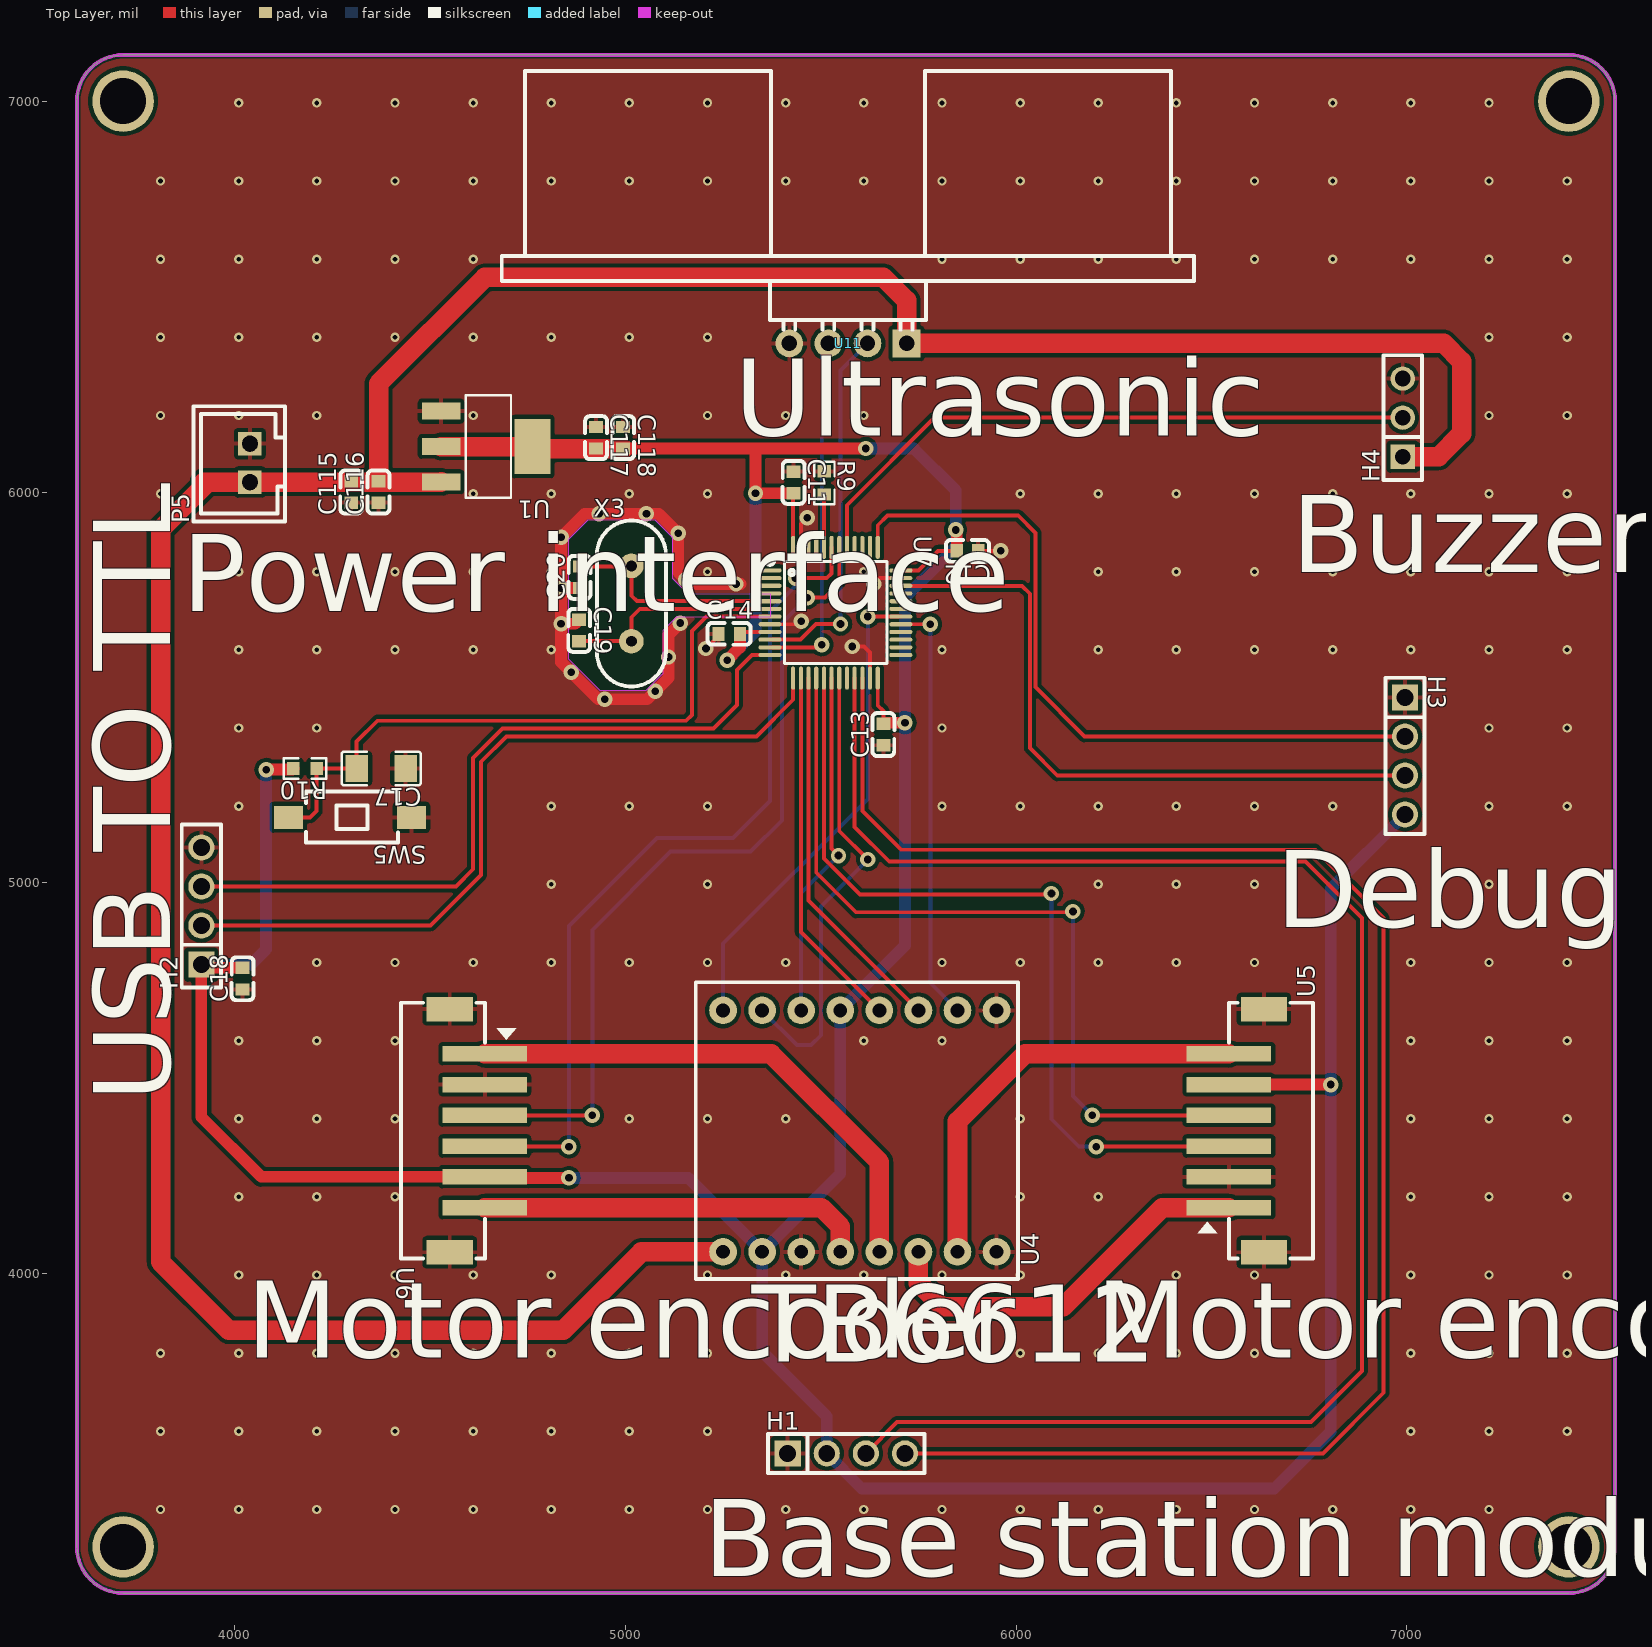
[diagram p0: Top Layer view]
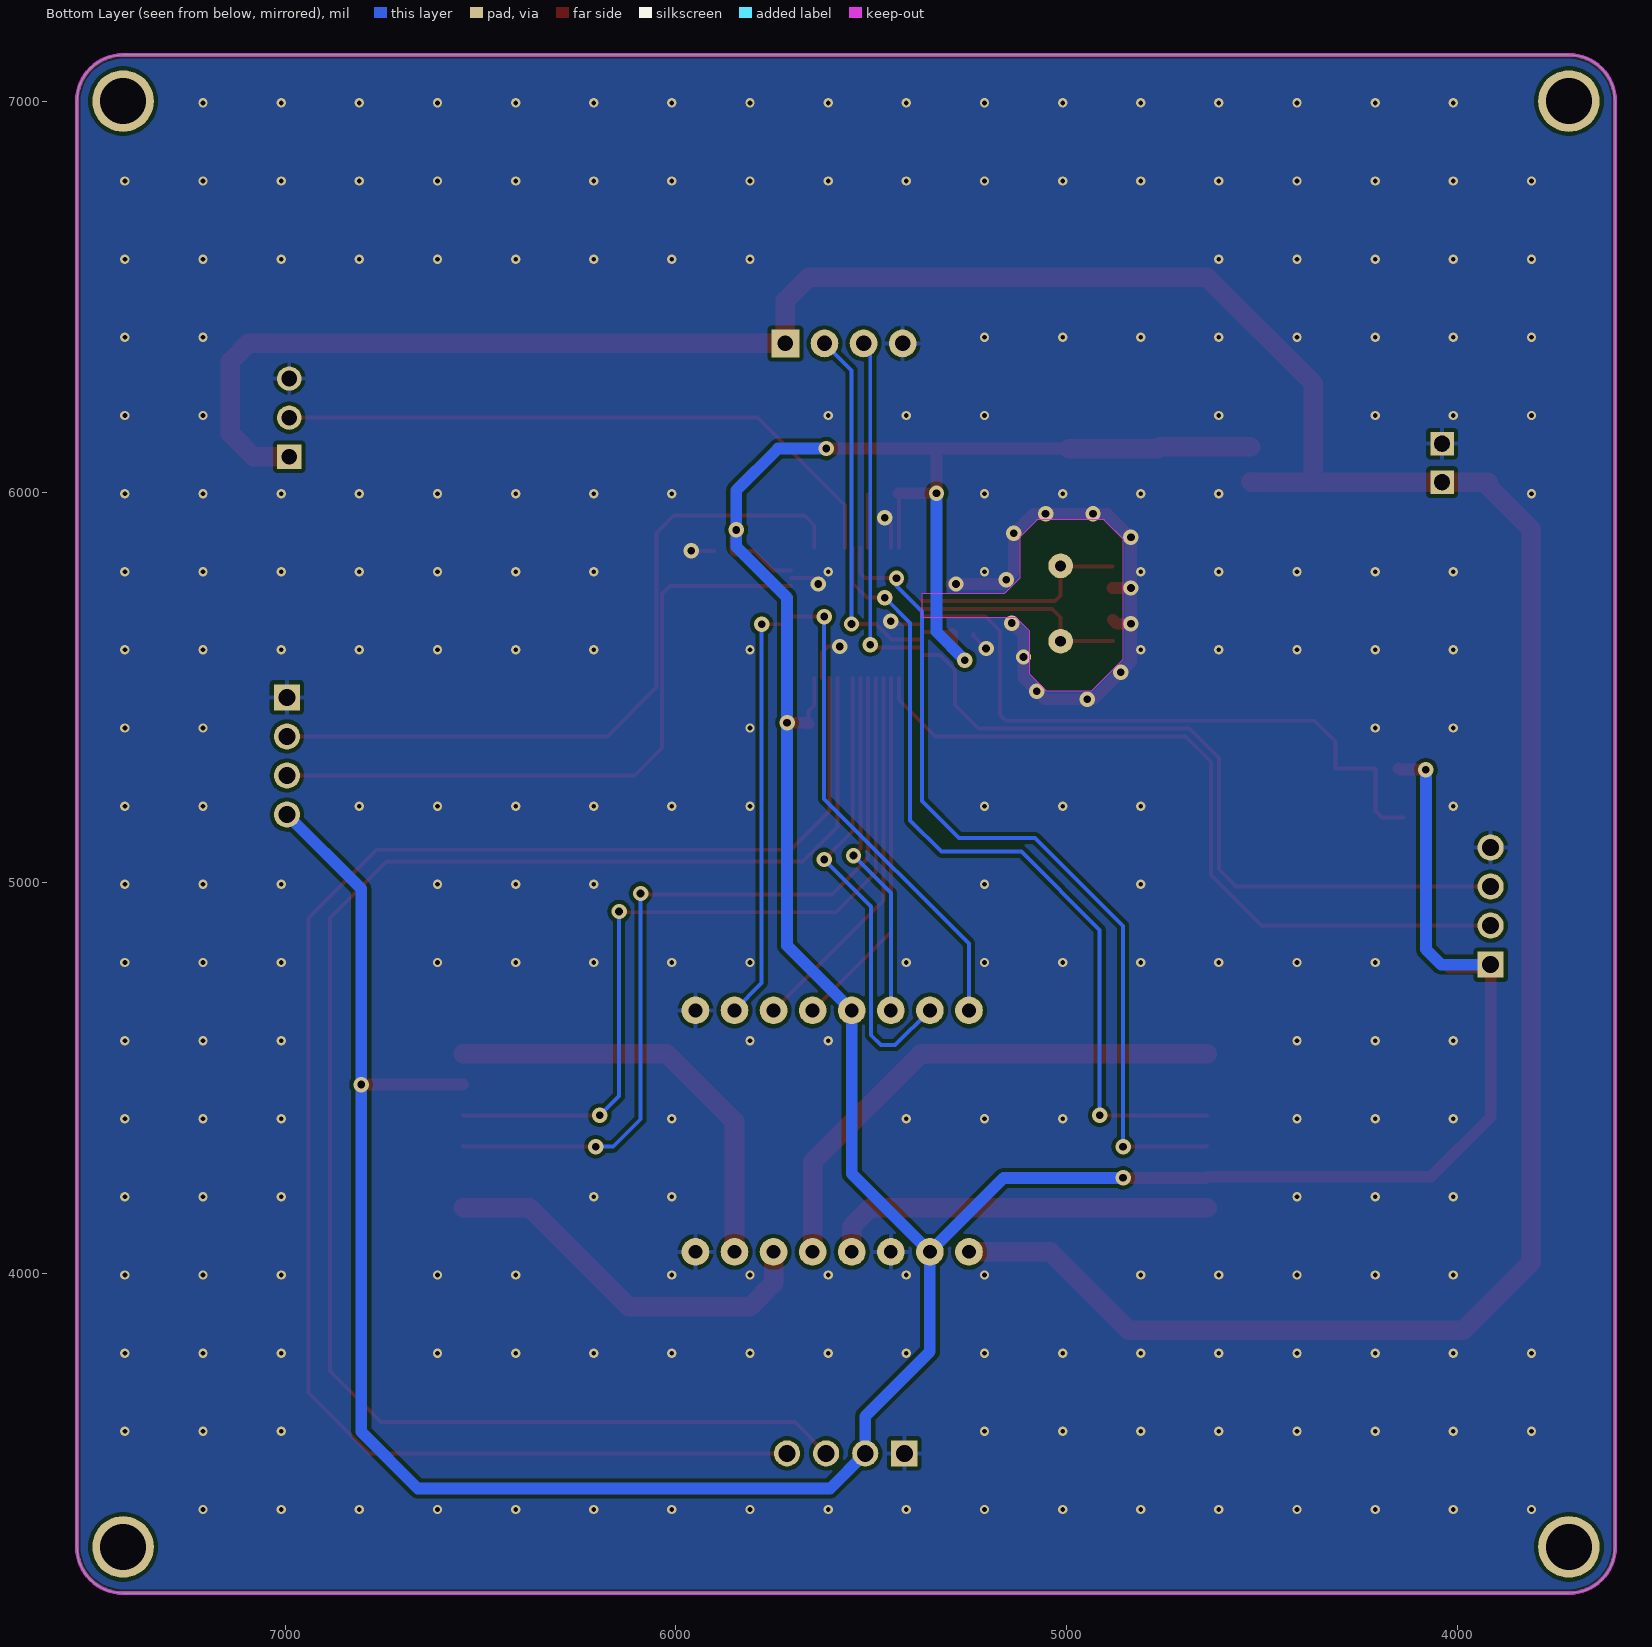
[diagram p1: Bottom Layer view, seen from below]
# Altium PCB MISC61262.pcbdoc
Units mil, origin at the board's own origin, x right, y up, seen from the top; angles counter-clockwise.
Board outline 3937.01 x 3937.01 mil, 2 copper layers (Top Layer, Bottom Layer), stack 62.206 mil thick; 27 components, 45 nets, 141 pads, 278 vias.

## Layer stack, top to bottom
Top Solder Mask Layer: solder mask 0.394, Dk 3.3
Top Layer: signal copper 1.379
Dielectric1: surface 59.449, FR4, Dk 4.5
Bottom Layer: signal copper 1.378
Bottom Solder Mask Layer: solder mask 0.394, Dk 3.3

## Board outline
3595.71,3300.39 ccw(c3713.82,3300.39) 3713.82,3182.28 7414.61,3182.28 ccw(c7414.61,3300.39) 7532.72,3300.39 7532.72,7001.18 ccw(c7414.61,7001.18) 7414.61,7119.29 3713.82,7119.29 ccw(c3713.82,7001.18) 3595.71,7001.18

## Design rules (kind name [scope] priority, off if disabled: settings)
BoardOutlineClearance copperThickness2oz_1 [All] p2 off: genericclearance=7.99 ignorepadtopadclearanceinfootprint=FALSE except(0: Arc-SplitContinuation Track-SplitContinuation SMDPad-SplitContinuation THPad-SplitContinuation Via-SplitContinuation Fill-SplitContinuation Region-SplitContinuation Poly-SplitContinuation Text-SplitContinuation Hole-SplitContinuation; 5.98: Arc-CutoutEdge Track-CutoutEdge SMDPad-CutoutEdge THPad-CutoutEdge Via-CutoutEdge Text-CutoutEdge; 6.9: Hole-OutlineEdge Hole-CutoutEdge; 10: Poly-OutlineEdge Poly-CutoutEdge; 11.81: Arc-OutlineEdge Track-OutlineEdge SMDPad-OutlineEdge THPad-OutlineEdge Via-OutlineEdge Fill-OutlineEdge Region-OutlineEdge Text-OutlineEdge Fill-CutoutEdge Region-CutoutEdge)
BoardOutlineClearance Plane_innerPlane_1 [All] p4 off: genericclearance=4.02 ignorepadtopadclearanceinfootprint=FALSE except(0: Arc-SplitContinuation Track-SplitContinuation SMDPad-SplitContinuation THPad-SplitContinuation Via-SplitContinuation Fill-SplitContinuation Region-SplitContinuation Poly-SplitContinuation Text-SplitContinuation Hole-SplitContinuation; 5.98: Arc-CutoutEdge Track-CutoutEdge SMDPad-CutoutEdge THPad-CutoutEdge Via-CutoutEdge Text-CutoutEdge; 6.9: Hole-OutlineEdge Hole-CutoutEdge; 10: Poly-OutlineEdge Poly-CutoutEdge; 11.81: Arc-OutlineEdge Track-OutlineEdge SMDPad-OutlineEdge THPad-OutlineEdge Via-OutlineEdge Fill-OutlineEdge Region-OutlineEdge Text-OutlineEdge Fill-CutoutEdge Region-CutoutEdge)
BoardOutlineClearance Copper_copperRegion_1 [All] p6 off: genericclearance=4.02 ignorepadtopadclearanceinfootprint=FALSE except(0: Arc-SplitContinuation Track-SplitContinuation SMDPad-SplitContinuation THPad-SplitContinuation Via-SplitContinuation Fill-SplitContinuation Region-SplitContinuation Poly-SplitContinuation Text-SplitContinuation Hole-SplitContinuation; 5.98: Arc-CutoutEdge Track-CutoutEdge SMDPad-CutoutEdge THPad-CutoutEdge Via-CutoutEdge Text-CutoutEdge; 6.9: Hole-OutlineEdge Hole-CutoutEdge; 10: Poly-OutlineEdge Poly-CutoutEdge; 11.81: Arc-OutlineEdge Track-OutlineEdge SMDPad-OutlineEdge THPad-OutlineEdge Via-OutlineEdge Fill-OutlineEdge Region-OutlineEdge Text-OutlineEdge Fill-CutoutEdge Region-CutoutEdge)
BoardOutlineClearance Copper_copperRegion_copperThickness1oz_1 [All] p8 off: genericclearance=4.02 ignorepadtopadclearanceinfootprint=FALSE except(0: Arc-SplitContinuation Track-SplitContinuation SMDPad-SplitContinuation THPad-SplitContinuation Via-SplitContinuation Fill-SplitContinuation Region-SplitContinuation Poly-SplitContinuation Text-SplitContinuation Hole-SplitContinuation; 5.98: Arc-CutoutEdge Track-CutoutEdge SMDPad-CutoutEdge THPad-CutoutEdge Via-CutoutEdge Text-CutoutEdge; 6.9: Hole-OutlineEdge Hole-CutoutEdge; 10: Poly-OutlineEdge Poly-CutoutEdge; 11.81: Arc-OutlineEdge Track-OutlineEdge SMDPad-OutlineEdge THPad-OutlineEdge Via-OutlineEdge Fill-OutlineEdge Region-OutlineEdge Text-OutlineEdge Fill-CutoutEdge Region-CutoutEdge)
BoardOutlineClearance Copper_copperRegion_Copper_copperRegion_1 [All] p10 off: genericclearance=4.02 ignorepadtopadclearanceinfootprint=FALSE except(0: Arc-SplitContinuation Track-SplitContinuation SMDPad-SplitContinuation THPad-SplitContinuation Via-SplitContinuation Fill-SplitContinuation Region-SplitContinuation Poly-SplitContinuation Text-SplitContinuation Hole-SplitContinuation; 5.98: Arc-CutoutEdge Track-CutoutEdge SMDPad-CutoutEdge THPad-CutoutEdge Via-CutoutEdge Text-CutoutEdge; 6.9: Hole-OutlineEdge Hole-CutoutEdge; 10: Poly-OutlineEdge Poly-CutoutEdge; 11.81: Arc-OutlineEdge Track-OutlineEdge SMDPad-OutlineEdge THPad-OutlineEdge Via-OutlineEdge Fill-OutlineEdge Region-OutlineEdge Text-OutlineEdge Fill-CutoutEdge Region-CutoutEdge)
BoardOutlineClearance copperThickness1oz_1 [All] p12: genericclearance=4.02 ignorepadtopadclearanceinfootprint=FALSE except(0: Arc-SplitContinuation Track-SplitContinuation SMDPad-SplitContinuation THPad-SplitContinuation Via-SplitContinuation Fill-SplitContinuation Region-SplitContinuation Poly-SplitContinuation Text-SplitContinuation Hole-SplitContinuation; 5.98: Arc-CutoutEdge Track-CutoutEdge SMDPad-CutoutEdge THPad-CutoutEdge Via-CutoutEdge Text-CutoutEdge; 6.9: Hole-OutlineEdge Hole-CutoutEdge; 10: Poly-OutlineEdge Poly-CutoutEdge; 11.81: Arc-OutlineEdge Track-OutlineEdge SMDPad-OutlineEdge THPad-OutlineEdge Via-OutlineEdge Fill-OutlineEdge Region-OutlineEdge Text-OutlineEdge Fill-CutoutEdge Region-CutoutEdge)
Clearance copperThickness2oz [All] p1 off: gap=7.99 ignorepadtopadclearanceinfootprint=FALSE except(5.98: SMDPad-Track SMDPad-SMDPad THPad-Track SMDPad-THPad THPad-THPad Track-Via SMDPad-Via THPad-Via Via-Via Fill-SMDPad Region-SMDPad Fill-THPad Region-THPad Fill-Via Region-Via Fill-Fill Fill-Region Region-Region Arc-Track Arc-SMDPad Arc-THPad Arc-Via Fill-Arc Region-Arc Arc-Arc Text-Track SMDPad-Text Text-THPad Text-Via Fill-Text Region-Text Arc-Text Text-Text; 6.9: Hole-Track Hole-SMDPad Hole-THPad Hole-Via Fill-Hole Region-Hole Hole-Arc Hole-Text; 10: Poly-Track Poly-SMDPad Poly-THPad Poly-Via Poly-Fill Poly-Region Poly-Poly Poly-Arc Poly-Text Poly-Hole; 11.81: Fill-Track Region-Track)
Clearance Plane_innerPlane [All] p3 off: gap=4.02 ignorepadtopadclearanceinfootprint=FALSE except(5.98: SMDPad-Track SMDPad-SMDPad THPad-Track SMDPad-THPad THPad-THPad Track-Via SMDPad-Via THPad-Via Via-Via Fill-SMDPad Region-SMDPad Fill-THPad Region-THPad Fill-Via Region-Via Fill-Fill Fill-Region Region-Region Arc-Track Arc-SMDPad Arc-THPad Arc-Via Fill-Arc Region-Arc Arc-Arc Text-Track SMDPad-Text Text-THPad Text-Via Fill-Text Region-Text Arc-Text Text-Text; 6.9: Hole-Track Hole-SMDPad Hole-THPad Hole-Via Fill-Hole Region-Hole Hole-Arc Hole-Text; 10: Poly-Track Poly-SMDPad Poly-THPad Poly-Via Poly-Fill Poly-Region Poly-Poly Poly-Arc Poly-Text Poly-Hole; 11.81: Fill-Track Region-Track)
Clearance Copper_copperRegion [All] p5 off: gap=4.02 ignorepadtopadclearanceinfootprint=FALSE except(5.98: SMDPad-Track SMDPad-SMDPad THPad-Track SMDPad-THPad THPad-THPad Track-Via SMDPad-Via THPad-Via Via-Via Fill-SMDPad Region-SMDPad Fill-THPad Region-THPad Fill-Via Region-Via Fill-Fill Fill-Region Region-Region Arc-Track Arc-SMDPad Arc-THPad Arc-Via Fill-Arc Region-Arc Arc-Arc Text-Track SMDPad-Text Text-THPad Text-Via Fill-Text Region-Text Arc-Text Text-Text; 6.9: Hole-Track Hole-SMDPad Hole-THPad Hole-Via Fill-Hole Region-Hole Hole-Arc Hole-Text; 10: Poly-Track Poly-SMDPad Poly-THPad Poly-Via Poly-Fill Poly-Region Poly-Poly Poly-Arc Poly-Text Poly-Hole; 11.81: Fill-Track Region-Track)
Clearance Copper_copperRegion_copperThickness1oz [All] p7 off: gap=4.02 ignorepadtopadclearanceinfootprint=FALSE except(5.98: SMDPad-Track SMDPad-SMDPad THPad-Track SMDPad-THPad THPad-THPad Track-Via SMDPad-Via THPad-Via Via-Via Fill-SMDPad Region-SMDPad Fill-THPad Region-THPad Fill-Via Region-Via Fill-Fill Fill-Region Region-Region Arc-Track Arc-SMDPad Arc-THPad Arc-Via Fill-Arc Region-Arc Arc-Arc Text-Track SMDPad-Text Text-THPad Text-Via Fill-Text Region-Text Arc-Text Text-Text; 6.9: Hole-Track Hole-SMDPad Hole-THPad Hole-Via Fill-Hole Region-Hole Hole-Arc Hole-Text; 10: Poly-Track Poly-SMDPad Poly-THPad Poly-Via Poly-Fill Poly-Region Poly-Poly Poly-Arc Poly-Text Poly-Hole; 11.81: Fill-Track Region-Track)
Clearance Copper_copperRegion_Copper_copperRegion [All] p9 off: gap=4.02 ignorepadtopadclearanceinfootprint=FALSE except(5.98: SMDPad-Track SMDPad-SMDPad THPad-Track SMDPad-THPad THPad-THPad Track-Via SMDPad-Via THPad-Via Via-Via Fill-SMDPad Region-SMDPad Fill-THPad Region-THPad Fill-Via Region-Via Fill-Fill Fill-Region Region-Region Arc-Track Arc-SMDPad Arc-THPad Arc-Via Fill-Arc Region-Arc Arc-Arc Text-Track SMDPad-Text Text-THPad Text-Via Fill-Text Region-Text Arc-Text Text-Text; 6.9: Hole-Track Hole-SMDPad Hole-THPad Hole-Via Fill-Hole Region-Hole Hole-Arc Hole-Text; 10: Poly-Track Poly-SMDPad Poly-THPad Poly-Via Poly-Fill Poly-Region Poly-Poly Poly-Arc Poly-Text Poly-Hole; 11.81: Fill-Track Region-Track)
Clearance copperThickness1oz [All] p11: gap=4.02 ignorepadtopadclearanceinfootprint=FALSE except(5.98: SMDPad-Track SMDPad-SMDPad THPad-Track SMDPad-THPad THPad-THPad Track-Via SMDPad-Via THPad-Via Via-Via Fill-SMDPad Region-SMDPad Fill-THPad Region-THPad Fill-Via Region-Via Fill-Fill Fill-Region Region-Region Arc-Track Arc-SMDPad Arc-THPad Arc-Via Fill-Arc Region-Arc Arc-Arc Text-Track SMDPad-Text Text-THPad Text-Via Fill-Text Region-Text Arc-Text Text-Text; 6.9: Hole-Track Hole-SMDPad Hole-THPad Hole-Via Fill-Hole Region-Hole Hole-Arc Hole-Text; 10: Poly-Track Poly-SMDPad Poly-THPad Poly-Via Poly-Fill Poly-Region Poly-Poly Poly-Arc Poly-Text Poly-Hole; 11.81: Fill-Track Region-Track)
DiffPairsRouting differentialPair [All] p1: maxlimit=6 minlimit=6 mostfreqgap=6 toplayer_minwidth=5 toplayer_prefwidth=10 toplayer_maxwidth=100 toplayer_mingap=6 toplayer_prefgap=6 toplayer_maxgap=6 bottomlayer_minwidth=5 bottomlayer_prefwidth=10 bottomlayer_maxwidth=100 bottomlayer_mingap=6 bottomlayer_prefgap=6 bottomlayer_maxgap=6 maxuncoupledlength=10
HoleToHoleClearance otherClearance [All] p1: gap=11.81 allowstackedmicrovias=TRUE
Length netLength [All] p1: minlimit=0 maxlimit=0
PasteMaskExpansion pasteMaskExpansion [All] p1: expansion=0
PlaneConnect innerPlane [All] p1: planeconnectstyle=Relief reliefexpansion=20 reliefentries=4 reliefconductorwidth=10 reliefairgap=10
PolygonConnect copperRegion_copperThickness1oz [All] p1 off: connectstyle=Relief reliefconductorwidth=10 reliefentries=4 polygonreliefangle="90 Angle" airgapwidth=10 via.connectstyle=Relief via.reliefconductorwidth=10 via.reliefentries=4 via.polygonreliefangle="90 Angle" via.airgapwidth=10
PolygonConnect copperRegion_Copper_copperRegion [All] p2 off: connectstyle=Relief reliefconductorwidth=10 reliefentries=4 polygonreliefangle="90 Angle" airgapwidth=10 via.connectstyle=Relief via.reliefconductorwidth=10 via.reliefentries=4 via.polygonreliefangle="90 Angle" via.airgapwidth=10
PolygonConnect copperRegion [All] p3: connectstyle=Relief reliefconductorwidth=10 reliefentries=4 polygonreliefangle="90 Angle" airgapwidth=10 via.connectstyle=Relief via.reliefconductorwidth=10 via.reliefentries=4 via.polygonreliefangle="90 Angle" via.airgapwidth=10
RoutingVias viaSize [All] p1: holewidth=12.01 width=24.02 viastyle="Through Hole" minholewidth=11.81 minwidth=19.68 maxholewidth=248.03 maxwidth=393.7
SolderMaskExpansion solderMaskExpansion [IsVia] p1: expansion=-1000 istentingtop=TRUE
SolderMaskExpansion solderMaskExpansion [All] p2: expansion=2 istentingtop=FALSE
Width copperThickness2oz_2 [All] p1 off: maxlimit=100 minlimit=8 preferedwidth=10
Width copperThickness1oz_2 [All] p2: maxlimit=100 minlimit=5 preferedwidth=10

## Components (designator, comment, footprint, x,y, rotation, side; value= is the part's Value field where it differs from the comment)
C11 "100nF" C0603 5430,6025 r270 top
C12 "100nF" C0603 5875,5850 r180 top
C13 "100nF" C0603 5660,5380 r90 top
C14 "100nF" C0603 5265.23,5637.46 r0 top
C17 "100uF" C1206 4374.54,5292.81 r180 top
C18 "100nF" C0603 4020,4755 r90 top
C19 "20pF" C0603 4881.22,5646.25 r270 top
C20 "20pF" C0603 4882.56,5782.44 r90 top
C115 "10uF" C0603 4297.9,6000.79 r90 top
C116 "100nF" C0603 4367.9,6000.79 r90 top
C117 "100nF" C0603 4924.4,6139.33 r270 top
C118 "10uF" C0603 4993.89,6139.33 r270 top
H1 "" HDR-TH_4P-P2.54-V-M 5565,3540 r0 top
H2 "" HDR-TH_4P-P2.54-V-F 3914.21,4940.79 r90 top
H3 "" HDR-TH_4P-P2.54-V-M 6995,5325 r270 top
H4 "" HDR-TH_3P-P2.54-V-F 6989.21,6190.79 r90 top
P5 "XH2.54 straight socket-2P" CONN-TH_XH2.54-2P 4038.69,6075.01 r90 top
R9 "10kΩ" R0603 5508.66,6023.69 r270 top
R10 "1kΩ" R0603 4179.54,5292.81 r180 top
SW5 "TS-1101-C-W" SW-SMD_L6.0-W3.3-LS8.0 4294.54,5167.81 r180 top
U1 "AMS1117-3.3" SOT-223-3_L6.5-W3.4-P2.30-LS7.0-BR 4645.01,6116.93 r180 top
U4 "" tb6612 5249.55,4055.79 r90 top
U5 "MXPH-2.0-06P-LT1-0-A" CONN-SMD_6P-P2.00_MXPH-2.0-6P-LT1-0-A 6589.1,4365.79 r270 top
U6 "MXPH-2.0-06P-LT1-0-A" CONN-SMD_6P-P2.00_MXPH-2.0-6P-LT1-0-A 4595,4365.79 r90 top
U7 "STM32F103C8T6" LQFP-48_L7.0-W7.0-P0.50-LS9.0-BL 5537.18,5691.49 r270 top
U11 "HC-SR04" TH_HC-SR04V 5569.21,6380.79 r180 top
X3 "8MHz" OSC-TH_L10.0-W4.5-P5.00 5015,5715 r0 top

## Footprints (in the part's own frame and the unit in brackets; to place one, negate y for a bottom-side part, rotate by r counter-clockwise, add the part's x,y. Pads: shape width x height; smd on the part's side, far side on the other; paste and mask are expansions set on the pad)
C0603 [mm]
  rect 0.8x0.9 smd: 1(-0.7,0) 2(0.7,0)
  silkscreen extent -1.41,-0.71 1.39,0.72
C1206 [mm]
  rect 1.485x1.728 smd paste-100 mask+0.051: 1(-1.593,0) 2(1.593,0)
  silkscreen extent -2.56,-1.09 2.56,1.09
CONN-SMD_6P-P2.00_MXPH-2.0-6P-LT1-0-A [mm]
  rect 1x5.5 smd paste+0 mask+0.05: 1(5,-1.14) 2(3,-1.14) 3(1,-1.14) 4(-1,-1.14) 5(-3,-1.14) 6(-5,-1.14)
  rect 1.6x3 smd paste+0 mask+0.05: 7(-7.9,1.14) 8(7.9,1.14)
  silkscreen extent -8.32,-3.17 8.32,4.32
CONN-TH_XH2.54-2P [mil]
  rect 60x60 hole 39.37 slot 41.34 at 0 deg paste+0 mask+1.97: 1(-49.22,0) 2(49.21,0)
  silkscreen extent -150,-90 145,145
HDR-TH_3P-P2.54-V-F [mil]
  rect 62x62 hole 40.16: 1(-100,0)
  round 62 hole 40.16: 2(0,0) 3(100,0)
  silkscreen extent -160,-49 160,49
HDR-TH_4P-P2.54-V-F [mm]
  rect 1.7x1.7 hole 1.1: 1(-3.81,0)
  round 1.7 hole 1.1: 2(-1.27,0) 3(1.27,0) 4(3.81,0)
  silkscreen extent -5.29,-1.27 5.29,1.27
HDR-TH_4P-P2.54-V-M [mm]
  rect 1.7x1.7 hole 1.1: 1(-3.81,0)
  round 1.7 hole 1.1: 2(-1.27,0) 3(1.27,0) 4(3.81,0)
  silkscreen extent -5.08,-1.27 5.08,1.27
LQFP-48_L7.0-W7.0-P0.50-LS9.0-BL [mm]
  oval 0.27x1.5 smd paste+0 mask+0.05: 1(-2.75,-4.25) 2(-2.25,-4.25) 3(-1.75,-4.25) 4(-1.25,-4.25) 5(-0.75,-4.25) 6(-0.25,-4.25) 7(0.25,-4.25) 8(0.75,-4.25) 9(1.25,-4.25) 10(1.75,-4.25) 11(2.25,-4.25) 12(2.75,-4.25) 25(2.75,4.25) 26(2.25,4.25) 27(1.75,4.25) 28(1.25,4.25) 29(0.75,4.25) 30(0.25,4.25) 31(-0.25,4.25) 32(-0.75,4.25) 33(-1.25,4.25) 34(-1.75,4.25) 35(-2.25,4.25) 36(-2.75,4.25)
  oval 1.5x0.27 smd paste+0 mask+0.05: 13(4.25,-2.75) 14(4.25,-2.25) 15(4.25,-1.75) 16(4.25,-1.25) 17(4.25,-0.75) 18(4.25,-0.25) 19(4.25,0.25) 20(4.25,0.75) 21(4.25,1.25) 22(4.25,1.75) 23(4.25,2.25) 24(4.25,2.75) 37(-4.25,2.75) 38(-4.25,2.25) 39(-4.25,1.75) 40(-4.25,1.25) 41(-4.25,0.75) 42(-4.25,0.25) 43(-4.25,-0.25) 44(-4.25,-0.75) 45(-4.25,-1.25) 46(-4.25,-1.75) 47(-4.25,-2.25) 48(-4.25,-2.75)
  silkscreen extent -3.59,-4.46 3.3,3.34
OSC-TH_L10.0-W4.5-P5.00 [mm]
  round 1.6 hole 0.7: 1(0,2.45) 2(0,-2.45)
  silkscreen extent -2.25,-5.39 2.25,5.39
R0603 [mil]
  rect 31.75x34.02 smd paste-3937.01 mask+2: 1(-29.66,0) 2(29.66,0)
  silkscreen extent -55,-26 55,26
SOT-223-3_L6.5-W3.4-P2.30-LS7.0-BR [mm]
  rect 2.5x1.1 smd: 1(2.97,-2.3) 2(2.97,0) 3(2.97,2.3)
  rect 2.34x3.6 smd: 4(-2.97,0)
  silkscreen extent -1.57,-3.33 1.37,3.33
SW-SMD_L6.0-W3.3-LS8.0 [mm]
  rect 1.9x1.5 smd: 1(-4,0) 2(4,0)
  silkscreen extent -3.14,-1.67 2.86,1.63
tb6612 [mm]
  round 1.8 hole 0.9: 1(0,0) 2(0,-2.54) 3(0,-5.08) 4(0,-7.62) 5(0,-10.16) 6(0,-12.7) 7(0,-15.24) 8(0,-17.78) 9(15.697,-17.78) 10(15.697,-15.24) 11(15.697,-12.7) 12(15.697,-10.16) 13(15.697,-7.62) 14(15.697,-5.08) 15(15.697,-2.54) 16(15.697,0)
  silkscreen extent -1.78,-19.18 17.53,1.78
TH_HC-SR04V [mm]
  rect 1.8x1.8 hole 1.001: 1(-3.81,0)
  round 1.8 hole 1.001: 2(-1.27,0) 3(1.27,0) 4(3.81,0)
  silkscreen extent -22.5,-17.7 22.5,-0.89

## Free pads (board coordinates)
  round 157.48 hole 118.11: 1(3713.82,7001.18) 1(3713.82,3300.39) 1(7414.61,7001.18) 1(7414.61,3300.39)

## Via types
v1: diameter 24.02, hole 12, Top Layer to Bottom Layer, 237 vias
v2: diameter 39.37, hole 19.7, Top Layer to Bottom Layer, 41 vias

## Nets (pads, with @x,y where several pads share a name; then routed paths per layer and width w, separated by ;. In a path a pad name is that pad's centre, name@x,y a point inside that pad or via, vN(x,y) a via of type N, cw(c..) or ccw(c..) an arc to the next point about the centre after c; other vN are vias at no path point)
+5V: C115.2 C116.2 H4.1 P5.1 U1.3 U4.1 U11.1 | length 7882.3
  Top Layer w50: 3920,6015 3810,5905 3810,4030 3985,3855 4840,3855 5040.79,4055.79 U4.1 ; 3920,6025.79 P5.1 4527.49,6025.79 U1.3 ; C116.2 4367.9,6277.9 4640,6550 5660,6550 5719.21,6490.79 U11.1 7094.21,6380.79 7140,6335 7140,6150 7080.79,6090.79 H4.1
AO1: U4.4 U6.6 | length 994.4
  Top Layer w50: U6.6 5501.06,4168.94 5549.55,4120.45 U4.4
AO2: U4.5 U6.1 | length 1354.1
  Top Layer w50: U6.1 5372.36,4562.64 5649.55,4285.45 U4.5
BO1: U4.7 U5.6 | length 1100.1
  Top Layer w50: U4.7 5849.55,4389.55 6022.64,4562.64 U5.6
BO2: U4.6 U5.1 | length 1005.2
  Top Layer w50: U4.6 5749.55,3975.45 5810,3915 6120,3915 6373.94,4168.94 U5.1
BOOT0: R9.2 U7.44 | length 135.6
  Top Layer w10: U7.44 5507.65,5993.01 R9.2
BOOT1: U7.20
CLK: H3.2 U7.37 | length 1881.8
  Top Layer w10: U7.37 5645.45,5915.45 5670,5940 6005,5940 6049.02,5895.98 6049.02,5500.98 6175,5375 H3.2
DIO: H3.3 U7.34 | length 1722.9
  Top Layer w10: U7.34 6014.61,5760.39 6035,5740 6035,5345 6105,5275 H3.3
GND: C11.1 C12.1 C13.1 C14.1 C17.1 C18.1 C19.1 C20.1 C115.1 C116.1 C117.1 C118.1 H1.1 H2.4 H3.1 H4.3 P5.2 R9.1 SW5.1 U1.1 U4.3 U4.8 U4.9 U5.2 U5.7 U5.8 U6.2 U6.7 U6.8 U7.8 U7.23 U7.35 U7.47 U11.4 | length 1993.4
  Top Layer w10: v2(5205.67,5600) 5237.68,5632.01 C14.1 ; U7.8 5441.96,5661.96 v2(5450,5670) ; U7.47 5448.6,5918.6 v2(5465,5935) ; v2(5580,5605) 5610,5605 5625.76,5589.24 U7.23 ; v2(5635,5765) 5650.07,5780.07 U7.35 ; C12.1 v2(5960,5850)
  Top Layer w30: C19.1 4870.74,5663.33 v2(4835,5663.33) ; C20.1 4882.42,5754.74 v2(4835,5754.74) ; v2(5140,5665) 5110,5635 v2(5110,5578.32) 5110,5525 v2(5075.79,5490.79) 5055,5470 4930,5470 v2(4861.04,5538.96) 4835,5565 v2(4835,5663.33) ; v2@5295,5765 5165,5765 5135,5795 v2(5135,5895) 5085,5945 v2(5053.36,5945) v2(4932.07,5945) 4895,5945 v2(4835,5885) v2(4835,5754.74) ; v2(4835,5663.33) v2(4835,5754.74)
  other v1: 3809.81,3396.38 4009.81,3396.38 4209.81,3396.38 4409.81,3396.38 4609.81,3396.38 4809.81,3396.38 5009.81,3396.38 5209.81,3396.38 5409.81,3396.38 5609.81,3396.38 5809.81,3396.38 6009.81,3396.38 6209.81,3396.38 6409.81,3396.38 6609.81,3396.38 6809.81,3396.38 7009.81,3396.38 7209.81,3396.38 3809.81,3596.38 4009.81,3596.38 4209.81,3596.38 4409.81,3596.38 4609.81,3596.38 4809.81,3596.38 5009.81,3596.38 5209.81,3596.38 7009.81,3596.38 7209.81,3596.38 7409.81,3596.38 3809.81,3796.38 4009.81,3796.38 4209.81,3796.38 4409.81,3796.38 4609.81,3796.38 4809.81,3796.38 5009.81,3796.38 5209.81,3796.38 5409.81,3796.38 5609.81,3796.38 5809.81,3796.38 6009.81,3796.38 6209.81,3796.38 6409.81,3796.38 6609.81,3796.38 7009.81,3796.38 7209.81,3796.38 7409.81,3796.38 4009.81,3996.38 4209.81,3996.38 4409.81,3996.38 4609.81,3996.38 4809.81,3996.38 5209.81,3996.38 5409.81,3996.38 5609.81,3996.38 5809.81,3996.38 6009.81,3996.38 6409.81,3996.38 6609.81,3996.38 7009.81,3996.38 7209.81,3996.38 7409.81,3996.38 4009.81,4196.38 4209.81,4196.38 4409.81,4196.38 6009.81,4196.38 6209.81,4196.38 7009.81,4196.38 7209.81,4196.38 7409.81,4196.38 4009.81,4396.38 4209.81,4396.38 4409.81,4396.38 5009.81,4396.38 5209.81,4396.38 5409.81,4396.38 6009.81,4396.38 7009.81,4396.38 7209.81,4396.38 7409.81,4396.38 4009.81,4596.38 4209.81,4596.38 4409.81,4596.38 5609.81,4596.38 5809.81,4596.38 7009.81,4596.38 7209.81,4596.38 7409.81,4596.38 4209.81,4796.38 4409.81,4796.38 4609.81,4796.38 4809.81,4796.38 5009.81,4796.38 5209.81,4796.38 5409.81,4796.38 5809.81,4796.38 6009.81,4796.38 6209.81,4796.38 6409.81,4796.38 6609.81,4796.38 7009.81,4796.38 7209.81,4796.38 7409.81,4796.38 4809.81,4996.38 5209.81,4996.38 6209.81,4996.38 6409.81,4996.38 6609.81,4996.38 7009.81,4996.38 7209.81,4996.38 7409.81,4996.38 4009.81,5196.38 4809.81,5196.38 5009.81,5196.38 5209.81,5196.38 5809.81,5196.38 6009.81,5196.38 6209.81,5196.38 6409.81,5196.38 6609.81,5196.38 6809.81,5196.38 7209.81,5196.38 7409.81,5196.38 4009.81,5396.38 4209.81,5396.38 5809.81,5396.38 7209.81,5396.38 7409.81,5396.38 4009.81,5596.38 4209.81,5596.38 4409.81,5596.38 4609.81,5596.38 4809.81,5596.38 5809.81,5596.38 6209.81,5596.38 6409.81,5596.38 6609.81,5596.38 6809.81,5596.38 7009.81,5596.38 7209.81,5596.38 7409.81,5596.38 4009.81,5796.38 4209.81,5796.38 4409.81,5796.38 4609.81,5796.38 4809.81,5796.38 5209.81,5796.38 5609.81,5796.38 6209.81,5796.38 6409.81,5796.38 6609.81,5796.38 6809.81,5796.38 7009.81,5796.38 7209.81,5796.38 7409.81,5796.38 3809.81,5996.38 4609.81,5996.38 4809.81,5996.38 5009.81,5996.38 5209.81,5996.38 6009.81,5996.38 6209.81,5996.38 6409.81,5996.38 6609.81,5996.38 6809.81,5996.38 7009.81,5996.38 7209.81,5996.38 7409.81,5996.38 3809.81,6196.38 4009.81,6196.38 4209.81,6196.38 4609.81,6196.38 5209.81,6196.38 5409.81,6196.38 5609.81,6196.38 7209.81,6196.38 7409.81,6196.38 3809.81,6396.38 4009.81,6396.38 4209.81,6396.38 4409.81,6396.38 4609.81,6396.38 4809.81,6396.38 5009.81,6396.38 5209.81,6396.38 7209.81,6396.38 7409.81,6396.38 3809.81,6596.38 4009.81,6596.38 4209.81,6596.38 4409.81,6596.38 4609.81,6596.38 5809.81,6596.38 6009.81,6596.38 6209.81,6596.38 6409.81,6596.38 6609.81,6596.38 6809.81,6596.38 7009.81,6596.38 7209.81,6596.38 7409.81,6596.38 3809.81,6796.38 4009.81,6796.38 4209.81,6796.38 4409.81,6796.38 4609.81,6796.38 4809.81,6796.38 5009.81,6796.38 5209.81,6796.38 5409.81,6796.38 5609.81,6796.38 5809.81,6796.38 6009.81,6796.38 6209.81,6796.38 6409.81,6796.38 6609.81,6796.38 6809.81,6796.38 7009.81,6796.38 7209.81,6796.38 7409.81,6796.38 4009.81,6996.38 4209.81,6996.38 4409.81,6996.38 4609.81,6996.38 4809.81,6996.38 5009.81,6996.38 5209.81,6996.38 5409.81,6996.38 5609.81,6996.38 5809.81,6996.38 6009.81,6996.38 6209.81,6996.38 6409.81,6996.38 6609.81,6996.38 6809.81,6996.38 7009.81,6996.38 7209.81,6996.38
  other v2: 4947,5470 5282.78,5765 5153.97,5776.03
OSC-IN: C20.2 U7.5 X3.1 | length 570.1
  Top Layer w10: C20.2 5013.54,5810 X3.1 5015,5735 5028.98,5721.02 U7.5
OSC-OUT: C19.2 U7.6 X3.2 | length 559
  Top Layer w10: C19.2 5014.85,5618.69 X3.2 5015,5680 5036.33,5701.33 U7.6
PA0: U7.10 U11.2 | length 943.6
  Top Layer w10: U7.10 5447.59,5622.59 5487.59,5662.59 v2(5550,5662.59)
  Bottom Layer w10: v2(5550,5662.59) 5550,6311.57 U11.2
PA1: U7.11 U11.3 | length 913.1
  Top Layer w10: U7.11 5495.16,5602.91 v2(5502.09,5609.84)
  Bottom Layer w10: v2(5502.09,5609.84) 5502.09,6363.66 U11.3
PA2: H2.3 U7.12 | length 1920.7
  Top Layer w10: H2.3 4565.79,4990.79 4610,5035 4610,5320 4685,5395 5225,5395 5285,5455 5285,5545 5323.22,5583.22 U7.12
PA3: H2.2 U7.13 | length 1979.3
  Top Layer w10: H2.2 4500.79,4890.79 4630,5020 4630,5310 4695,5375 5335,5375 5428.91,5468.91 U7.13
PA4: U4.12 U7.14 | length 933.6
  Top Layer w10: U7.14 5448.6,4874.74 U4.12
PA5: U4.11 U7.15 | length 966.9
  Top Layer w10: U7.15 5468.28,4955.06 U4.11
PA6: U5.4 U7.16 | length 2088.9
  Top Layer w10: U7.16 5487.97,5027.03 5590,4925 6143.16,4925 v2(6145,4926.84) ; v2(6194.84,4405.16) U5.4
  Bottom Layer w10: v2(6145,4926.84) 6145,4455 v2(6194.84,4405.16)
PA7: U5.3 U7.17 | length 2145.4
  Top Layer w10: U7.17 5507.65,5062.35 5600,4970 6087.06,4970 v2(6090,4972.94) ; v2(6205,4325) 6542.8,4325 U5.3
  Bottom Layer w10: v2(6090,4972.94) 6090,4395 6160,4325 v2(6205,4325)
PA8: U4.10 U7.29 | length 1092.5
  Top Layer w10: U7.29 v2(5780,5661.96)
  Bottom Layer w10: v2(5780,5661.96) 5780,4743.34 U4.10
PA9: U4.16 U7.30 | length 1245.8
  Top Layer w10: v2(5620,5681.65) U7.30
  Bottom Layer w10: U4.16 5249.55,4844.55 5620,5215 v2(5620,5681.65)
PA10: U7.31
PA11: U7.32
PA12: U7.33
PA15: U7.38
PB0: U4.14 U7.18 | length 897.2
  Top Layer w10: U7.18 5527.34,5087.66 v2(5545,5070)
  Bottom Layer w10: U4.14 5449.55,4974.55 v2(5545,5070)
PB1: U4.15 U7.19 | length 1191.7
  Top Layer w10: U7.19 5547.02,5132.98 v2(5620,5060)
  Bottom Layer w10: U4.15 5438.34,4585 5475,4585 5500,4610 5500,4940 v2(5620,5060)
PB3: U7.39
PB4: U7.40
PB5: H4.2 U7.41 | length 1623.2
  Top Layer w10: U7.41 5566.71,5966.71 5790.79,6190.79 H4.2
PB6: U6.3 U7.42 | length 2137.2
  Top Layer w10: U6.3 4640.04,4405 v2(4915,4405) ; v2(5465,5730) 5510,5730 5547.02,5767.02 U7.42
  Bottom Layer w10: v2(4915,4405) 4915,4880 5115,5080 5320,5080 5400,5160 5400,5665 v2(5465,5730)
PB7: U6.4 U7.43 | length 2189.1
  Top Layer w10: U6.4 4641.3,4325 v2(4855,4325) ; v2(5435,5780) 5515,5780 5527.34,5792.34 U7.43
  Bottom Layer w10: v2(4855,4325) 4855,4890 5080,5115 5275,5115 5370,5210 5370,5695 5435,5760 v2(5435,5780)
PB8: U7.45
PB9: U7.46
PB10: H1.3 U7.21 | length 4292.7
  Top Layer w10: U7.21 5586.39,5143.61 5675,5055 6740,5055 6885,4910 6885,3750.32 6754.68,3620 5695,3620 H1.3
PB11: H1.4 U7.22 | length 4291.8
  Top Layer w10: U7.22 5606.08,5183.92 5705,5085 6765,5085 6940,4910 6940,3695 6785,3540 H1.4
PB12: U7.25
PB13: U7.26
PB14: U7.27
PB15: U7.28
PC13: U7.2
REST: C17.2 R10.1 SW5.2 U7.7 | length 1675.6
  Top Layer w10: SW5.2 4192.81,5167.81 4209.2,5184.2 R10.1 C17.2 4311.84,5361.84 4365,5415 5155,5415 5170,5430 5170,5645 5206.65,5681.65 U7.7
VBAT: U7.1
VCC: C11.2 C12.2 C13.2 C14.2 C18.2 C117.2 C118.2 H1.2 H2.1 H3.4 R10.2 U1.2 U1.4 U4.2 U4.13 U5.5 U6.5 U7.9 U7.24 U7.36 U7.48 | length 11564.7
  Top Layer w10: C14.2 5297.61,5642.28 U7.9 ; U7.48 5428.91,5996.35 C11.2 ; U7.24 5645.45,5454.55 5660,5440 C13.2 ; U7.36 5749.76,5799.76 5800,5850 C12.2
  Top Layer w30: C18.2 3922.44,4782.56 H2.1 3914.21,4400.79 4067.32,4247.68 U6.5 4642.56,4245 v2(4855,4245) ; v2(4080,5290) 4147.07,5290 R10.2 ; C118.2 5332.56,6111.77 ; v2(5260,5570) 5292.8,5602.8 C14.2 ; C11.2 v2(5332.56,5997.44) 5332.56,6111.77 ; v2(5615,6111.77) 5332.56,6111.77 ; C13.2 5662.44,5410 v2(5715,5410) ; v2(5845,5903.47) 5847.44,5901.03 C12.2 ; U5.5 v2(6805,4483.9)
  Top Layer w50: U1.2 U1.4 4767.1,6111.77 C117.2 C118.2
  Bottom Layer w30: H2.1 4040.79,4790.79 4080,4830 v2(4080,5290) ; v2(4855,4245) 5160.34,4245 U4.2 ; v2(5260,5570) 5332.56,5642.56 v2(5332.56,5997.44) ; v2(5615,6111.77) 5738.23,6111.77 5845,6005 v2(5845,5903.47) 5845,5860 5715,5730 v2(5715,5410) 5715,4839.24 U4.13 5549.55,4255.79 U4.2 ; H3.4 6805,4985 v2(6805,4483.9) 6805,3595 6660,3450 5605,3450 H1.2 5515,3635 5349.55,3800.45 U4.2
pads on no net: U7.3 U7.4

## Polygon pours and split planes (outlines as drawn)
GND on Bottom Layer (solid, remove dead copper, pour order 2): 3525,7245 3525,3080 7700,3080 7700,7245
GND on Top Layer (solid, remove dead copper, pour order 2): 3000,7415 3000,3000 7930,3000 7930,7415

## Keep-outs
Board Outline Layer:
  region: 5369.86,5740.7 5369.86,5681.65 5368.2,5680 5130,5680 5095,5645 5095,5535 5051.37,5491.37 4934.88,5491.37 4854.39,5571.86 4854.39,5879.39 4905,5930 5075,5930 5120,5885 5120,5780 5159.3,5740.7
  lines w10: 3595.71,3300.39 ccw(c3713.82,3300.39) 3713.82,3182.28 7414.61,3182.28 ccw(c7414.61,3300.39) 7532.72,3300.39 7532.72,7001.18 ccw(c7414.61,7001.18) 7414.61,7119.29 3713.82,7119.29 ccw(c3713.82,7001.18) 3595.71,7001.18 3595.71,3300.39

## Silkscreen, mask and mechanical layers (free items; w line width, h text height)
Top Silkscreen Layer:
  text "Ultrasonic" at 5280,6145 h196.85
  text "Buzzer" at 6705,5795 h196.85
  text "Power interface" at 3865,5695 h196.85
  text "Debug interface" at 6666,4886.28 h196.85
  text "USB TO TTL" at 3835,4440 h196.85 r90
  text "Motor encoder" at 4030,3785 h196.85
  text "Motor encoder" at 6205,3785 h196.85
  text "TB6612" at 5322.7,3774.86 h196.85
  text "Base station module" at 5200,3225 h196.85